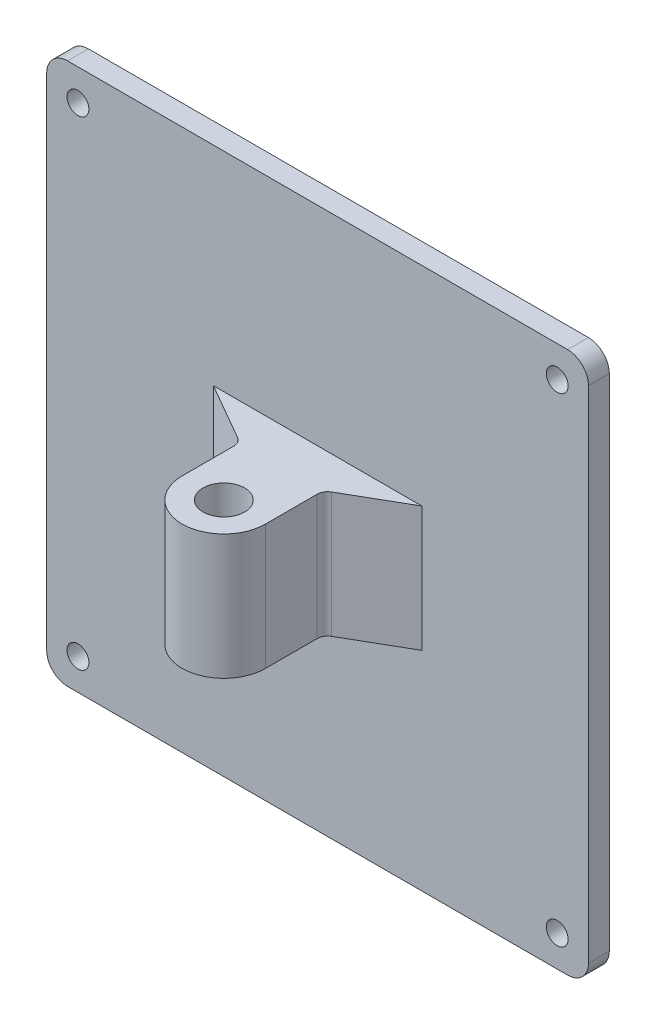
SolidWorks part; units mm, degrees
material "普通碳钢"
ref_plane "前视基准面" through (0, 0, 0) normal (0, 0, 1) x (1, 0, 0)
ref_plane "上视基准面" through (0, 0, 0) normal (0, 1, 0) x (1, 0, 0)
ref_plane "右视基准面" through (0, 0, 0) normal (1, 0, 0) x (0, 0, -1)
sketch "草图1" plane through (0, 0, 0) normal (0, 0, 1) x (1, 0, 0)
  line L1 (-120, -130) -> (120, -130)
  line L2 (-130, -120) -> (-130, 120)
  line L3 (-120, 130) -> (120, 130)
  line L4 (130, -120) -> (130, 120)
  line L5 (-130, -130) -> (130, 130) construction
  line L6 (-130, 130) -> (130, -130) construction
  line L7 (-115, -115) -> (115, -115) construction
  line L8 (-115, -115) -> (-115, 115) construction
  line L9 (-115, 115) -> (115, 115) construction
  line L10 (115, -115) -> (115, 115) construction
  line L11 (-115, -115) -> (115, 115) construction
  line L12 (-115, 115) -> (115, -115) construction
  circle A0 centre (-115, 115) radius 5.25
  circle A1 centre (115, 115) radius 5.25
  circle A2 centre (115, -115) radius 5.25
  circle A3 centre (-115, -115) radius 5.25
  arc A4 (-120, -130) -> (-130, -120) centre (-120, -120) cw
  arc A5 (120, -130) -> (130, -120) centre (120, -120) ccw
  arc A6 (120, 130) -> (130, 120) centre (120, 120) cw
  arc A7 (-130, 120) -> (-120, 130) centre (-120, 120) cw
  point P0 (0, 0)
  point P6 (0, 0)
  dimension "D3" = 10.5
  dimension "D6" = 10
  dimension "D1" = 260
  dimension "D2" = 260
  dimension "D4" = 230
  dimension "D5" = 230
extrude "凸台-拉伸1" add sketch "草图1" along normal blind 10
sketch "草图2" plane through (0, 0, 0) normal (0, 1, 0) x (1, 0, 0)
  line L6 (0, -5.5) -> (0, 5.5) construction
  line L8 (0, -10) -> (0, -43.1928) construction
  line L9 (-50, -10) -> (50, -10)
  line L10 (120, -10) -> (-120, -10) construction
  line L11 (-50, -10) -> (-20, -27.2789)
  line L12 (-20, -27.2789) -> (-20, -55)
  line L14 (20, -55) -> (20, -27.2789)
  line L15 (20, -27.2789) -> (50, -10)
  arc A1 (-20, -55) -> (20, -55) centre (0, -55) ccw
  dimension "D4" = 40
  dimension "D5" = 45
  dimension "D6" = 100
  dimension "D7" = 40
extrude "凸台-拉伸2" add sketch "草图2" along normal mid plane 60
sketch "草图3" plane through (0, -30, 0) normal (0, -1, 0) x (1, 0, 0)
  circle A0 centre (0, 55) radius 10
  point P3 (0, -45)
  point P4 (0, 55)
  dimension "D1" = 20
extrude "切除-拉伸1" cut sketch "草图3" against normal blind 134
fillet "圆角1" radius 5 2 edges at (20, 0, 27.2789) (-20, 0, 27.2789)
